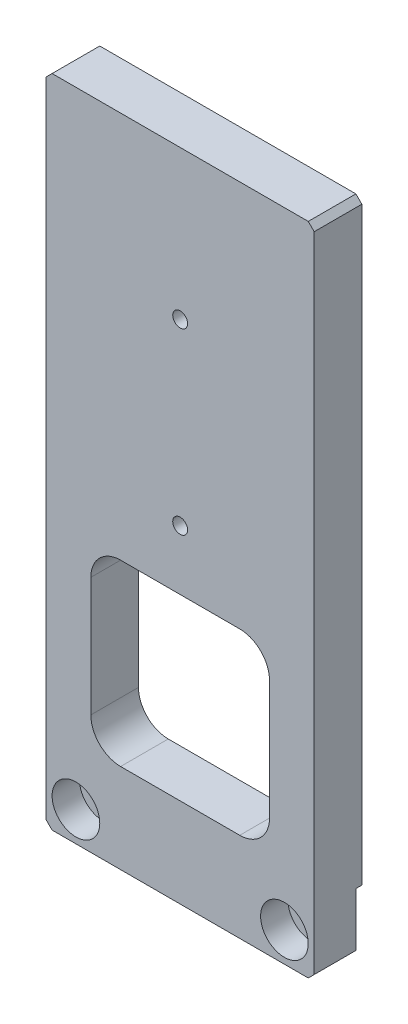
from build123d import *

# Parameters (mm, degrees)
SKETCH1_W                                          = 45
SKETCH1_H                                          = 110
BOSS_EXTRUDE1_DEPTH                                = 4
HOLE_SIZE_BASED_ON_SOCKET_HEAD_CAP_SCR_D           = 4.5
HOLE_SIZE_BASED_ON_SOCKET_HEAD_CAP_SCR_DEPTH       = 12.4
HOLE_SIZE_BASED_ON_SOCKET_HEAD_CAP_SCR_CBORE_D     = 8
HOLE_SIZE_BASED_ON_SOCKET_HEAD_CAP_SCR_CBORE_DEPTH = 4.6
HOLE_SIZE_BASED_ON_SOCKET_HEAD_CAP_SCR_TIP         = 1.351936393
SKETCH4_W                                          = 1
SKETCH4_H                                          = 10
CUT_EXTRUDE1_DEPTH                                 = 72.175838597
M3_TAPPED_HOLE1_D                                  = 2.5
CHAMFER1_SIZE                                      = 1
CUT_EXTRUDE2_DEPTH                                 = 60.960403601


with BuildPart() as part:
    # Sketch1 → Boss-Extrude1 (new, symmetric)
    with BuildSketch(Plane.XY):
        Rectangle(SKETCH1_W, SKETCH1_H)
    extrude(amount=BOSS_EXTRUDE1_DEPTH, both=True)

    # Hole size (% based on socket head cap screw type)1
    with Locations(Plane.XY.offset(4)):
        with Locations((-17.5, -50), (17.5, -50)):
            CounterBoreHole(HOLE_SIZE_BASED_ON_SOCKET_HEAD_CAP_SCR_D / 2, HOLE_SIZE_BASED_ON_SOCKET_HEAD_CAP_SCR_CBORE_D / 2, HOLE_SIZE_BASED_ON_SOCKET_HEAD_CAP_SCR_CBORE_DEPTH, depth=HOLE_SIZE_BASED_ON_SOCKET_HEAD_CAP_SCR_DEPTH)
            with Locations((0, 0, -(HOLE_SIZE_BASED_ON_SOCKET_HEAD_CAP_SCR_DEPTH + HOLE_SIZE_BASED_ON_SOCKET_HEAD_CAP_SCR_TIP / 2))):  # 118° drill point
                Cone(0, HOLE_SIZE_BASED_ON_SOCKET_HEAD_CAP_SCR_D / 2, HOLE_SIZE_BASED_ON_SOCKET_HEAD_CAP_SCR_TIP, mode=Mode.SUBTRACT)

    # Sketch4 → Cut-Extrude1 (cut, through all)
    with BuildSketch(Plane(origin=(22.5, 0, 0), x_dir=(0, 0, -1), z_dir=(1, 0, 0))):
        with Locations((3.5, -50)):
            Rectangle(SKETCH4_W, SKETCH4_H)
    extrude(amount=-CUT_EXTRUDE1_DEPTH, mode=Mode.SUBTRACT)

    # M3 Tapped Hole1 (through all)
    with Locations(Plane.XY.offset(4)):
        with Locations((0, 30), (0, 0)):
            Hole(M3_TAPPED_HOLE1_D / 2)

    # Chamfer1
    chamfer1_edges = [part.edges().sort_by_distance(p)[0] for p in [
        (22.5, -55, 0.5),
        (-22.5, -55, 0.5),
        (-22.5, 55, 0),
        (22.5, 55, 0),
    ]]
    chamfer(chamfer1_edges, length=CHAMFER1_SIZE)

    # Sketch7 → Cut-Extrude2 (cut, through all)
    with BuildSketch(Plane.XY.offset(4)):
        with BuildLine():
            Line((10, -10), (-10, -10))
            ThreePointArc((-10, -10), (-13.535533906, -11.464466094), (-15, -15))
            Line((-15, -15), (-15, -35))
            ThreePointArc((-15, -35), (-13.535533906, -38.535533906), (-10, -40))
            Line((-10, -40), (10, -40))
            ThreePointArc((10, -40), (13.535533906, -38.535533906), (15, -35))
            Line((15, -35), (15, -15))
            ThreePointArc((15, -15), (13.535533906, -11.464466094), (10, -10))
        make_face()
    extrude(amount=-CUT_EXTRUDE2_DEPTH, mode=Mode.SUBTRACT)


solid = part.part
